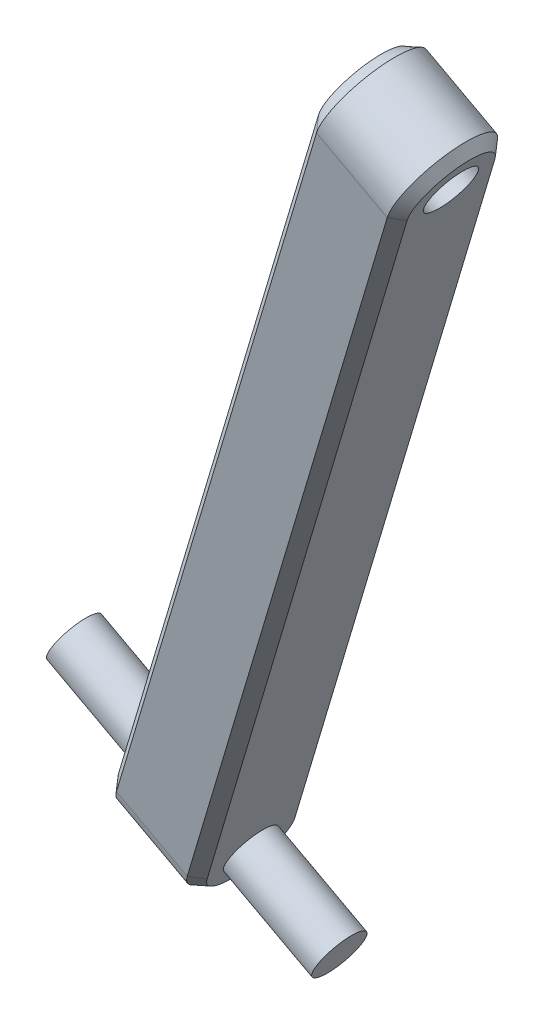
from build123d import *

# Parameters (mm, degrees)
BOSS_EXTRUDE1_DEPTH            = 5
F_2_5_2_5_DIAMETER_HOLE1_D     = 2.5
F_2_5_2_5_DIAMETER_HOLE1_DEPTH = 31.642263263
CHAMFER1_SIZE                  = 0.5


with BuildPart() as part:
    # Sketch1 → Boss-Extrude1 (new body)
    with BuildSketch(Plane(origin=(14.029336503, -7.536520805, 0), x_dir=(0.4732361692035663, 0.8809355981895235, 0), z_dir=(0.8809355981895235, -0.4732361692035663, -1.915856770880308e-15))):
        with BuildLine():
            Line((-90.390644299, -267.73860401), (-32.919543007, -250.502812288))
            ThreePointArc((-32.919543007, -250.502812288), (-31.243071775, -247.390025079), (-34.355858984, -245.713553847))
            Line((-34.355858984, -245.713553847), (-91.826960276, -262.949345569))
            ThreePointArc((-91.826960276, -262.949345569), (-93.503431508, -266.062132778), (-90.390644299, -267.73860401))
        make_face()
    extrude(amount=-BOSS_EXTRUDE1_DEPTH)

    # Sketch2 → Revolve1 (revolve)
    with BuildSketch(Plane.XY.offset(-265.34397479)):
        Polygon((-37.304454842, -81.963976858), (-37.896000054, -83.065146356), (-33.491322063, -85.431327202), (-32.899776851, -84.330157704), align=None)
    revolve(axis=Axis((-36.90956153, -83.595058405, -265.34397479), (0.880935598189524, -0.47323616920356526, 0)))

    # Sketch3 → Revolve2 (revolve)
    with BuildSketch(Plane.XY.offset(-265.34397479)):
        Polygon((-28.49509886, -86.69633855), (-29.086644072, -87.797508048), (-24.681966081, -90.163688894), (-24.090420869, -89.062519396), align=None)
    revolve(axis=Axis((-28.100205548, -88.327420097, -265.34397479), (0.8809355981895229, -0.4732361692035673, 0)))

    # Ø2.5 (2.5) Diameter Hole1
    with Locations(Plane(origin=(9.624658513, -5.170339959, 0), x_dir=(0, 0, 1), z_dir=(-0.8809355981895236, 0.4732361692035664, 1.9158567708803085e-15))):
        with Locations((-248.108183067, -33.637700995)):
            Hole(F_2_5_2_5_DIAMETER_HOLE1_D / 2, depth=F_2_5_2_5_DIAMETER_HOLE1_DEPTH)

    # Chamfer1
    chamfer1_edges = [part.edges().sort_by_distance(p)[0] for p in [
        (-5.160693088, -32.693474082, -247.390025079),
        (-20.23247849, -60.749808642, -254.331449708),
        (-34.624547222, -87.540841327, -266.062132778),
        (-15.827800499, -63.115989488, -254.331449708),
        (-0.756015097, -35.059654928, -247.390025079),
        (-15.148083829, -61.850687613, -259.120708149),
        (-30.219869231, -89.907022173, -266.062132778),
        (-19.55276182, -59.484506767, -259.120708149),
    ]]
    chamfer(chamfer1_edges, length=CHAMFER1_SIZE)


solid = part.part
